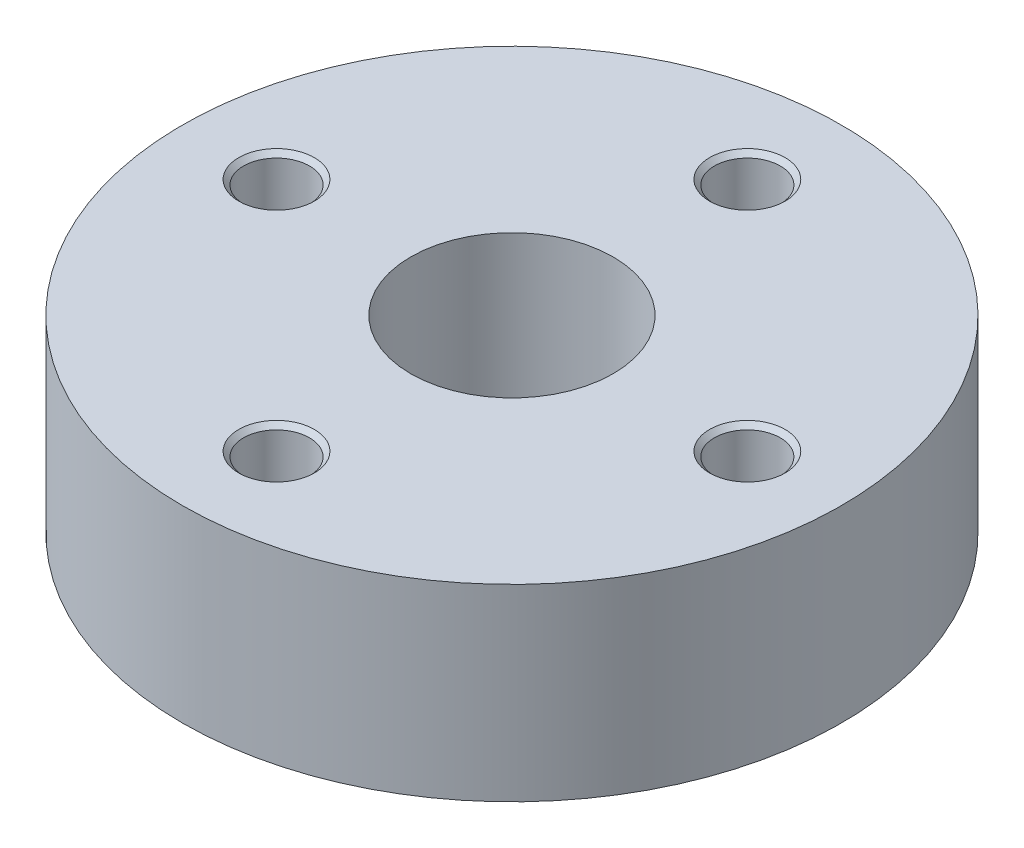
SolidWorks part; units mm, degrees
ref_plane "前视基准面" through (0, 0, 0) normal (0, 0, 1) x (1, 0, 0)
ref_plane "上视基准面" through (0, 0, 0) normal (0, 1, 0) x (1, 0, 0)
ref_plane "右视基准面" through (0, 0, 0) normal (1, 0, 0) x (0, 0, -1)
sketch "草图1" plane through (0, 0, 0) normal (0, 1, 0) x (1, 0, 0)
  circle A0 centre (0, 0) radius 70
  circle A1 centre (0, 0) radius 21.5
  dimension "D1" = 140
  dimension "D2" = 43
extrude "凸台-拉伸1" add sketch "草图1" along normal blind 40
hole_wizard "M16 螺纹孔1" positions "草图3" profile "草图4" tap size "M16" standard "GB"
sketch "草图3" plane through (0, 40, 0) normal (0, 1, 0) x (1, 0, 0)
  line L7 (0, 50) -> (0, -50) construction
  circle A0 centre (0, 0) radius 50 construction
  point P0 (0, 50)
  point P45 (50, 0)
  point P46 (0, -50)
  point P47 (-50, 0)
  dimension "D1" = 100
  dimension "D2" = 4
sketch "草图4" plane through (0, 40, -50) normal (1, 0, 0) x (0, 0, 1)
  line L0 (0, 0) -> (0, 32)
  line L1 (0, 32) -> (7, 27.794)
  line L2 (7, 27.794) -> (7, 1.025)
  line L3 (7, 1.025) -> (8.025, 0)
  line L5 (8.025, 0) -> (0, 0)
  line L6 (-7, 1.025) -> (-8.025, 0) construction
  line L10 (0, 32) -> (-7, 27.794) construction
  line L11 (0, -6.35) -> (0, 107.95) construction
  dimension "螺纹孔钻头直径" = 14
  dimension "螺纹孔钻头深度" = 32
  dimension "近端锥形沉头孔直径" = 16.05
  dimension "近端锥形沉头孔角度" = 90
  dimension "导头角度" = 118
cosmetic thread "孔螺蚊线1"
cosmetic thread "孔螺蚊线2"
cosmetic thread "孔螺蚊线3"
cosmetic thread "孔螺蚊线4"
hole_wizard "M16 螺纹孔3" positions "草图10" profile "草图11" tap size "M16" standard "GB"
sketch "草图10" plane through (0, 0, 0) normal (0, -1, 0) x (-1, 0, 0)
  line L0 (0, 0) -> (-35.3553, 35.3553) construction
  line L2 (0, 50) -> (0, -50) construction
  circle A0 centre (0, 0) radius 50 construction
  point P0 (-35.3553, 35.3553)
  point P16 (35.3553, 35.3553)
  point P17 (35.3553, -35.3553)
  point P18 (-35.3553, -35.3553)
  dimension "D1" = 45
  dimension "D2" = 4
sketch "草图11" plane through (35.3553, 0, -35.3553) normal (1, 0, 0) x (0, 0, -1)
  line L0 (0, 0) -> (0, 32)
  line L1 (0, 32) -> (7, 27.794)
  line L2 (7, 27.794) -> (7, 1.025)
  line L3 (7, 1.025) -> (8.025, 0)
  line L5 (8.025, 0) -> (0, 0)
  line L6 (-7, 1.025) -> (-8.025, 0) construction
  line L10 (0, 32) -> (-7, 27.794) construction
  line L11 (0, -6.35) -> (0, 107.95) construction
  dimension "螺纹孔钻头直径" = 14
  dimension "螺纹孔钻头深度" = 32
  dimension "近端锥形沉头孔直径" = 16.05
  dimension "近端锥形沉头孔角度" = 90
  dimension "导头角度" = 118
cosmetic thread "孔螺蚊线6"
cosmetic thread "孔螺蚊线7"
cosmetic thread "孔螺蚊线8"
cosmetic thread "孔螺蚊线9"
